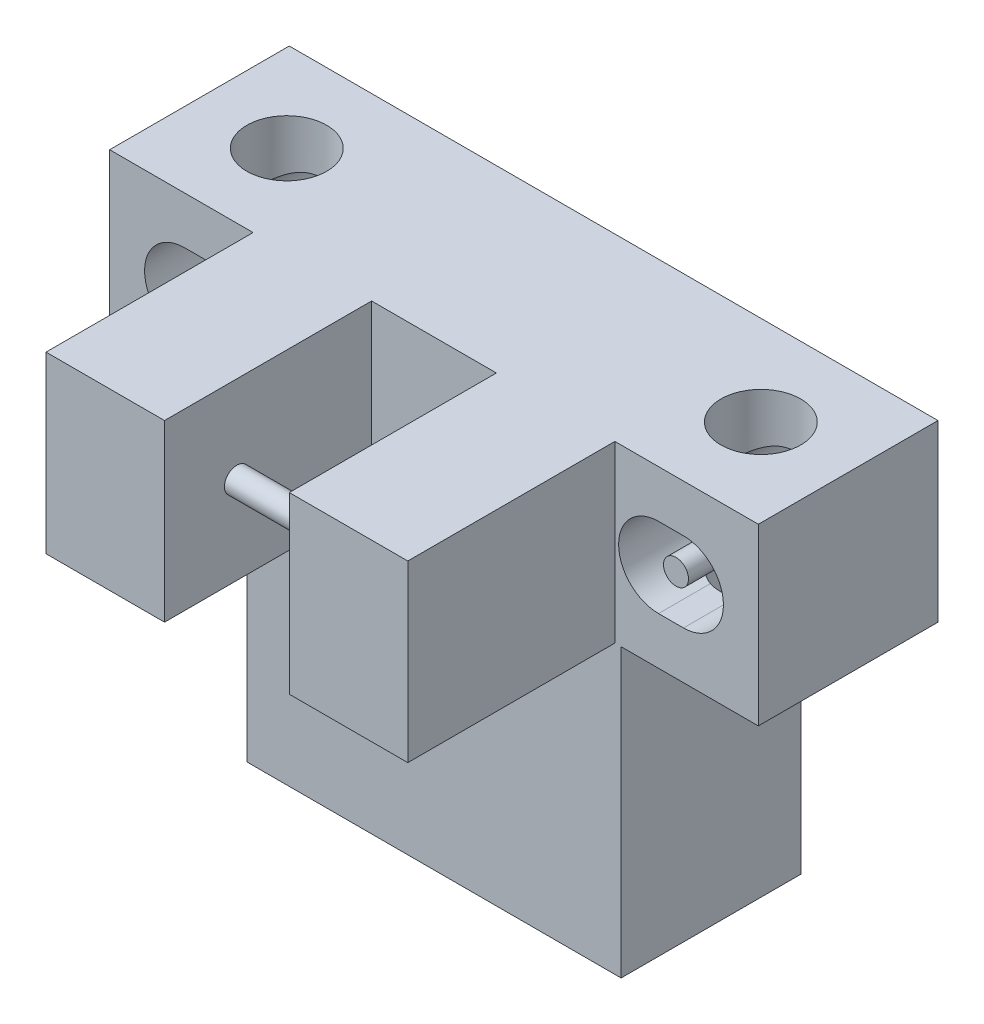
from build123d import *

# Parameters (mm, degrees)
EXTRUDE_1_DEPTH         = 3.6
SKETCH_2_W              = 4.75
SKETCH_2_H              = 7
EXTRUDE_2_DEPTH         = 8.3
SKETCH_3_R              = 0.5
EXTRUDE_3_DEPTH         = 9
HOLE_WIZARD_3_2_3_2_1_D = 3.2
SKETCH_4_R              = 0.5
EXTRUDE_4_DEPTH         = 7
EXTRUDE_4_2_DEPTH       = 7


with BuildPart() as part:
    # 草图1 → 凸台-拉伸1 (new, symmetric)
    with BuildSketch(Plane.XY):
        Polygon((13, 18.5), (-13, 18.5), (-13, 11.5), (-7.5, 11.5), (-7.5, 0), (7.5, 0), (7.5, 11.5), (13, 11.5), align=None)
        with BuildLine():
            Line((-10, 16.6), (-9, 16.6))
            ThreePointArc((-9, 16.6), (-7.4, 15), (-9, 13.4))
            Line((-9, 13.4), (-10, 13.4))
            ThreePointArc((-10, 13.4), (-11.6, 15), (-10, 16.6))
        make_face(mode=Mode.SUBTRACT)
        with BuildLine():
            Line((10, 16.6), (9, 16.6))
            ThreePointArc((9, 16.6), (7.4, 15), (9, 13.4))
            Line((9, 13.4), (10, 13.4))
            ThreePointArc((10, 13.4), (11.6, 15), (10, 16.6))
        make_face(mode=Mode.SUBTRACT)
    extrude(amount=EXTRUDE_1_DEPTH, both=True)

    # 草图2 → 凸台-拉伸2 (add)
    with BuildSketch(Plane.XY.offset(3.6)):
        with Locations((-4.875, 15)):
            Rectangle(SKETCH_2_W, SKETCH_2_H)
        with Locations((4.875, 15)):
            Rectangle(SKETCH_2_W, SKETCH_2_H)
    extrude(amount=EXTRUDE_2_DEPTH)

    # 草图3 → 凸台-拉伸3 (add)
    with BuildSketch(Plane(origin=(-2.5, 0, 0), x_dir=(0, 0, -1), z_dir=(1, 0, 0))):
        with Locations(Location((-9, 15, 0), (0, 0, 270))):
            Circle(SKETCH_3_R)
    extrude(amount=EXTRUDE_3_DEPTH)

    # Ø3.2 (3.2) 直径孔1 (through all)
    with Locations(Plane(origin=(0, 18.5, 0), x_dir=(1, 0, 0), z_dir=(0, 1, 0))):
        with Locations((-9.5, 0), (9.5, 0)):
            Hole(HOLE_WIZARD_3_2_3_2_1_D / 2)


with BuildPart() as body_2:
    # 草图4 → 凸台-拉伸4 (new body)
    with BuildSketch(Plane(origin=(0, 0, -3.6), x_dir=(-1, 0, 0), z_dir=(0, 0, -1))):
        with Locations((9.5, 15)):
            Circle(SKETCH_4_R)
    extrude(amount=-EXTRUDE_4_DEPTH)


with BuildPart() as body_3:
    # 草图4 → Extrude 4 2 (new body)
    with BuildSketch(Plane(origin=(0, 0, -3.6), x_dir=(-1, 0, 0), z_dir=(0, 0, -1))):
        with Locations(Location((-9.5, 15, 0), (0, 0, 180))):
            Circle(SKETCH_4_R)
    extrude(amount=-EXTRUDE_4_2_DEPTH)


solid = Compound([part.part, body_2.part, body_3.part])
